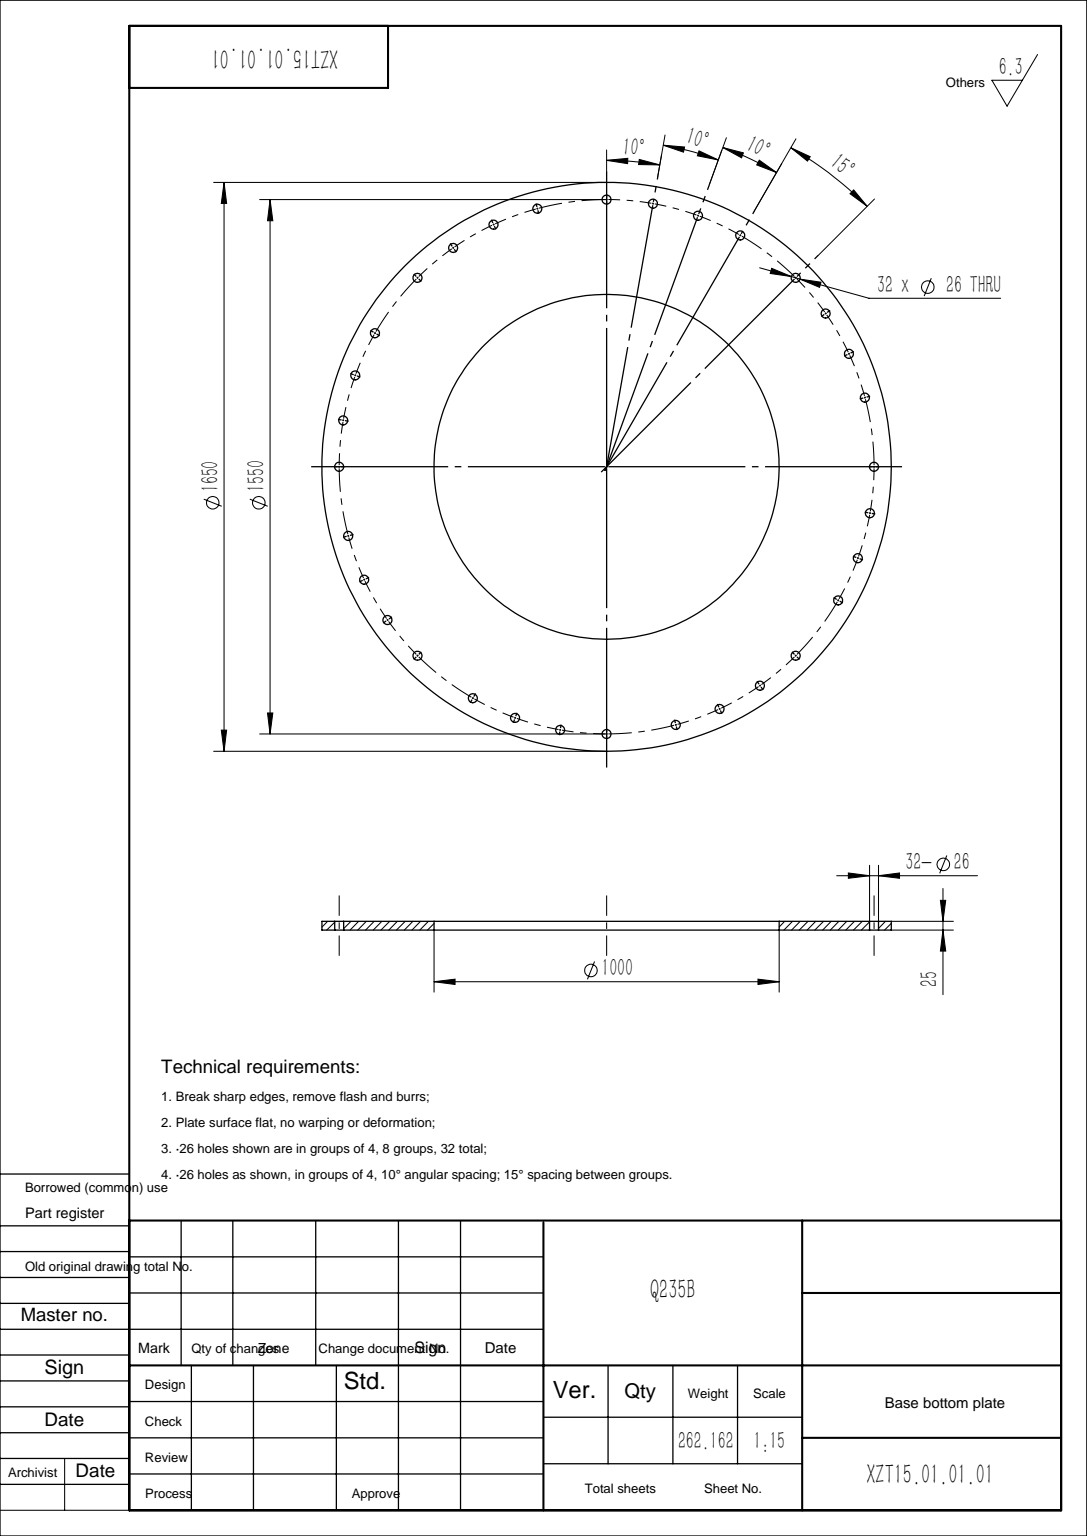
from build123d import *

# Parameters (mm, degrees)
SKETCH1_R                    = 825
SKETCH1_R_2                  = 500
BOSS_EXTRUDE1_DEPTH          = 25
F_24_5_24_5_DIAMETER_HOLE1_D = 26


with BuildPart() as part:
    # Sketch1 → Boss-Extrude1 (new body)
    with BuildSketch(Plane(origin=(0, 0, 0), x_dir=(1, 0, 0), z_dir=(0, 1, 0))):
        with Locations(Location((0, 0, 0), (0, 0, 270))):
            Circle(SKETCH1_R)
        with Locations(Location((0, 0, 0), (0, 0, 270))):
            Circle(SKETCH1_R_2, mode=Mode.SUBTRACT)
    extrude(amount=BOSS_EXTRUDE1_DEPTH)

    # Ø24.5 (24.5) Diameter Hole1 (through all)
    with Locations(Plane(origin=(0, 25, 0), x_dir=(1, 0, 0), z_dir=(0, 1, 0))):
        with Locations((0, 775), (134.577337692, 763.226008584), (265.065611077, 728.261781109), (387.5, 671.169687933), (548.00775542, 548.00775542), (634.842834324, 444.521738172), (702.388534953, 327.529152849), (748.592515374, 200.584759954), (775, 0), (763.226008584, -134.577337692), (728.261781109, -265.065611077), (671.169687933, -387.5), (548.00775542, -548.00775542), (444.521738172, -634.842834324), (327.529152849, -702.388534953), (200.584759954, -748.592515374), (0, -775), (-134.577337692, -763.226008584), (-265.065611077, -728.261781109), (-387.5, -671.169687933), (-548.00775542, -548.00775542), (-634.842834324, -444.521738172), (-702.388534953, -327.529152849), (-748.592515374, -200.584759954), (-775, 0), (-763.226008584, 134.577337692), (-728.261781109, 265.065611077), (-671.169687933, 387.5), (-548.00775542, 548.00775542), (-444.521738172, 634.842834324), (-327.529152849, 702.388534953), (-200.584759954, 748.592515374)):
            Hole(F_24_5_24_5_DIAMETER_HOLE1_D / 2)


solid = part.part
